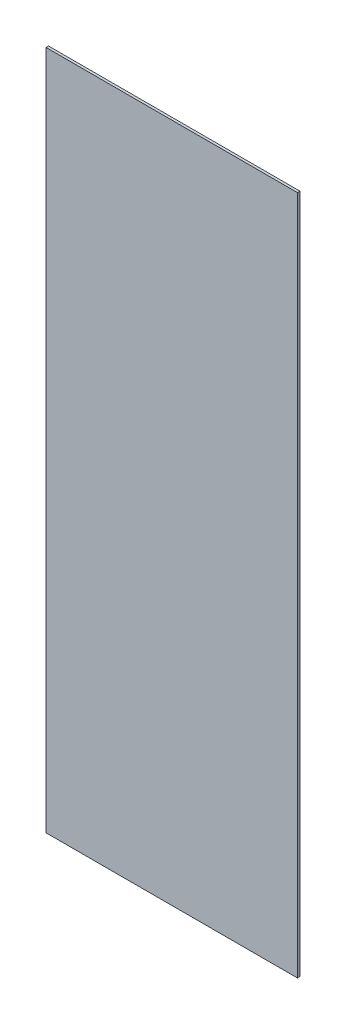
from build123d import *

# Parameters (mm, degrees)
SKETCH_1_W      = 499
SKETCH_1_H      = 1350
EXTRUDE_1_DEPTH = 5


with BuildPart() as part:
    # 草图1 → 凸台-拉伸1 (new body)
    with BuildSketch(Plane.XY):
        Rectangle(SKETCH_1_W, SKETCH_1_H)
    extrude(amount=EXTRUDE_1_DEPTH)


solid = part.part
